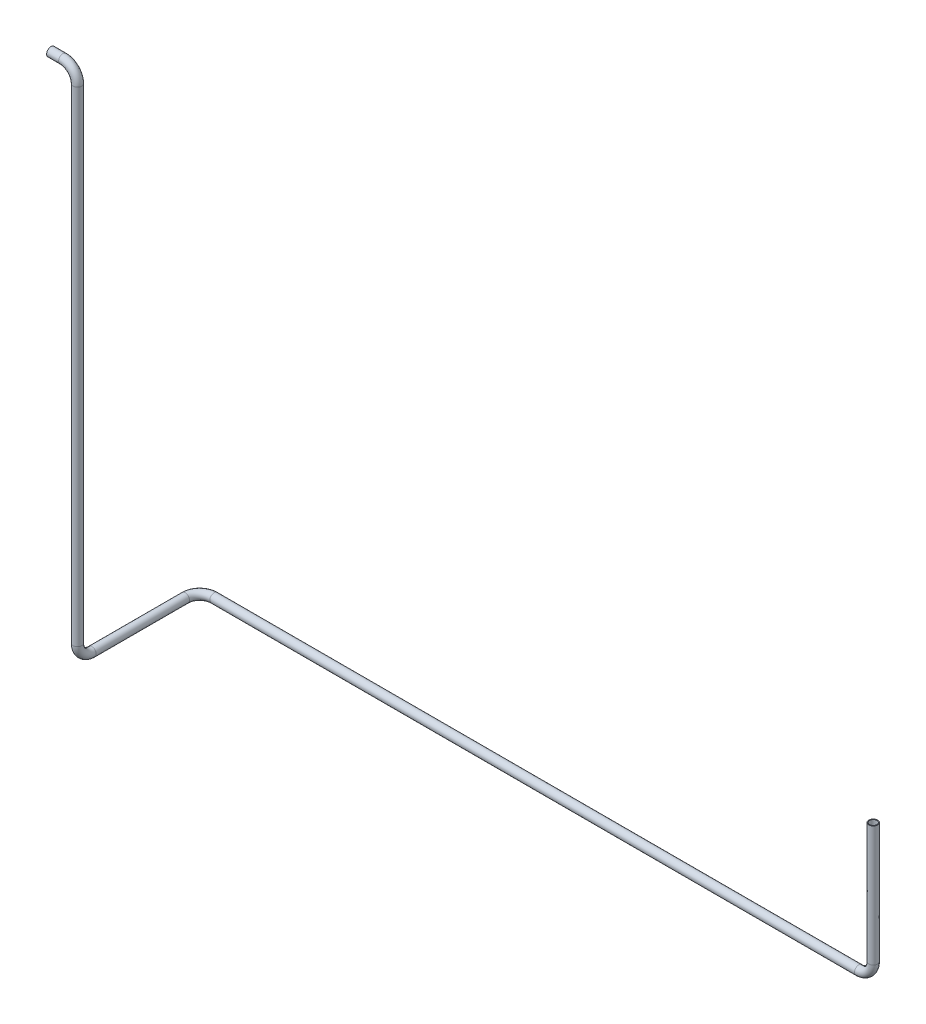
from build123d import *

# Parameters (mm, degrees)
SWEEP_1_PROFILE_R   = 6
SWEEP_1_PROFILE_R_2 = 5


with BuildPart() as part:
    # 扫描-薄件1: sweep along a curve in space
    with BuildLine() as sweep_1_path:
        Line((1880.512693362, 1112.598953747, 256.07159483), (1880.512693362, 1278.953453372, 256.07159483))
        ThreePointArc((1860.512693362, 1092.598953747, 256.07159483), (1874.654828986, 1098.456818123, 256.07159483), (1880.512693362, 1112.598953747, 256.07159483))
        Line((1860.512693362, 1092.598953747, 256.07159483), (969.949972589, 1092.598953747, 256.07159483))
        ThreePointArc((949.949972589, 1092.598953747, 276.07159483), (955.807836965, 1092.598953747, 261.929459206), (969.949972589, 1092.598953747, 256.07159483))
        Line((949.949972589, 1092.598953747, 276.07159483), (949.949972589, 1092.598953747, 404.912562332))
        ThreePointArc((949.949972589, 1092.598953747, 404.912562332), (949.949972589, 1098.456818123, 419.054697956), (949.949972589, 1112.598953747, 424.912562332))
        Line((949.949972589, 1112.598953747, 424.912562332), (949.949972589, 1782.095116422, 424.912562332))
        ThreePointArc((949.949972589, 1782.095116422, 424.912562332), (944.092108213, 1796.237252046, 424.912562332), (929.949972589, 1802.095116422, 424.912562332))
        Line((929.949972589, 1802.095116422, 424.912562332), (913.359234408, 1802.095116422, 424.912562332))
    # 扫描-薄件1 profile (on start of the path) → 扫描-薄件1 (sweep)
    with BuildSketch(Plane(origin=(913.359234408, 1802.095116422, 424.912562332), x_dir=(0, 0, 1), z_dir=(1, 0, 0))):
        Circle(SWEEP_1_PROFILE_R)
        Circle(SWEEP_1_PROFILE_R_2, mode=Mode.SUBTRACT)
    sweep(path=sweep_1_path.line)


solid = part.part
